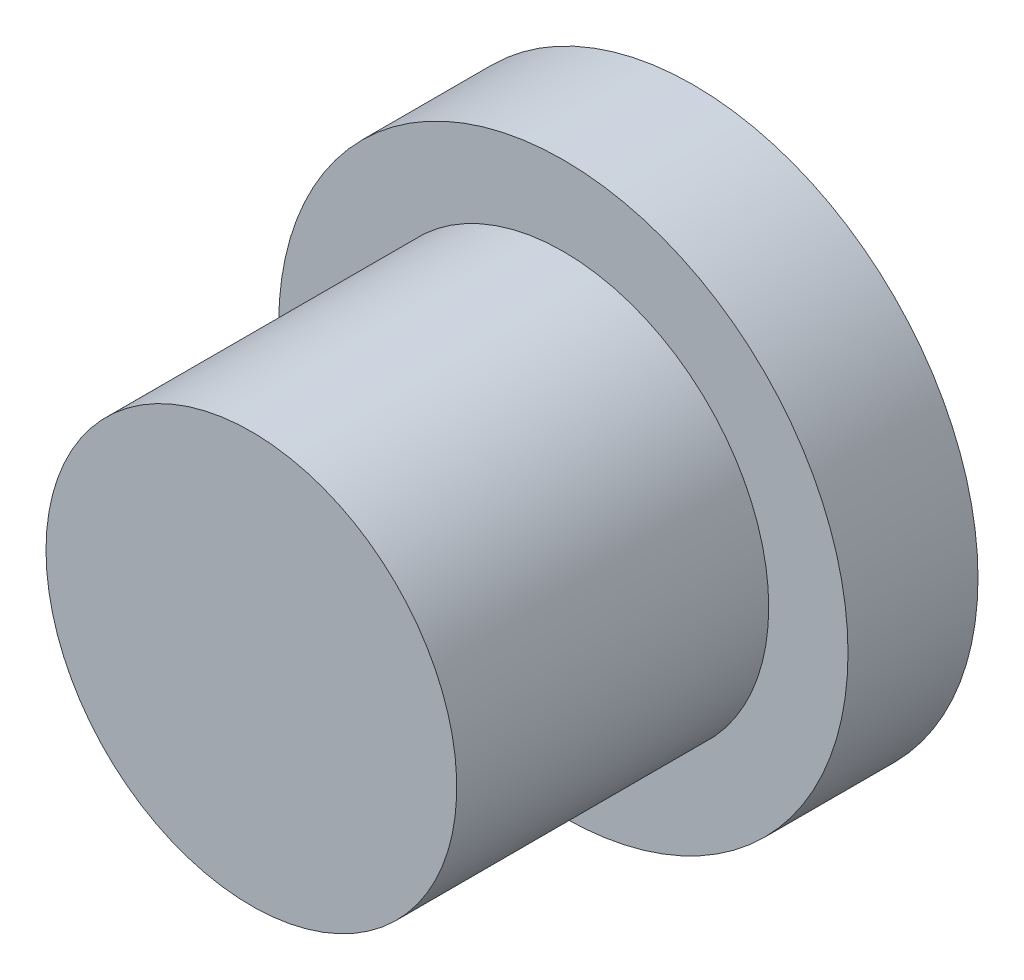
from build123d import *

# Parameters (mm, degrees)
SKETCH_1_R          = 10.95
EXTRUDE_1_DEPTH     = 5
SKETCH_2_R          = 7.9
EXTRUDE_2_DEPTH     = 17
CUT_EXTRUDE_1_DEPTH = 5


with BuildPart() as part:
    # 草图1 → 凸台-拉伸1 (new body)
    with BuildSketch(Plane.XY):
        Circle(SKETCH_1_R)
    extrude(amount=EXTRUDE_1_DEPTH)

    # 草图2 → 凸台-拉伸2 (add)
    with BuildSketch(Plane(origin=(0, 0, 0), x_dir=(-1, 0, 0), z_dir=(0, 0, -1))):
        Circle(SKETCH_2_R)
    extrude(amount=-EXTRUDE_2_DEPTH)

    # 草图3 → 切除-拉伸1 (cut)
    with BuildSketch(Plane(origin=(0, 0, 0), x_dir=(-1, 0, 0), z_dir=(0, 0, -1))):
        Polygon((0, 4.734272207), (-4.1, 2.367136104), (-4.1, -2.367136104), (0, -4.734272207), (4.1, -2.367136104), (4.1, 2.367136104), align=None)
    extrude(amount=-CUT_EXTRUDE_1_DEPTH, mode=Mode.SUBTRACT)


solid = part.part
